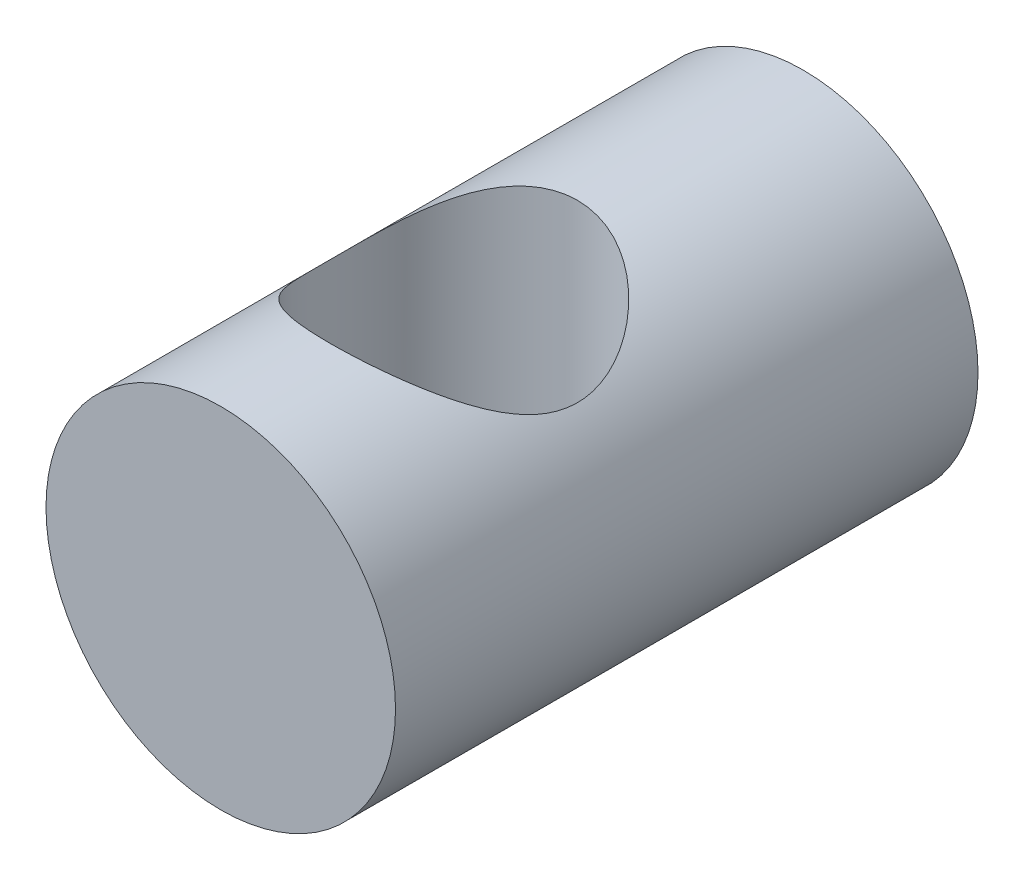
SolidWorks part; units mm, degrees
ref_plane "Front Plane" through (0, 0, 0) normal (0, 0, 1) x (1, 0, 0)
ref_plane "Top Plane" through (0, 0, 0) normal (0, 1, 0) x (1, 0, 0)
ref_plane "Right Plane" through (0, 0, 0) normal (1, 0, 0) x (0, 0, -1)
sketch "Sketch1" plane through (0, 0, 0) normal (0, 0, 1) x (1, 0, 0)
  circle A0 centre (0, 0) radius 6
  dimension "D1" = 12
extrude "Boss-Extrude1" add sketch "Sketch1" along normal blind 20
hole_wizard "M10 Tapped Hole2" positions "Sketch7" profile "Sketch5" tap size "M10" standard "Gb"
sketch "Sketch7" plane through (0, 0, 0) normal (0, 1, 0) x (1, 0, 0)
  line L0 (-6, -20) -> (6, -20) construction
  line L1 (6, -20) -> (6, 0) construction
  point P0 (0, -12)
  dimension "D1" = 8
  dimension "D2" = 6
cosmetic thread "CosmeticThread 2" parameters "D2"=10
sketch "Sketch5" plane through (0, 0, 12) normal (1, 0, 0) x (0, 0, -1)
  line L0 (0, 0) -> (0, 6)
  line L1 (0, 6) -> (4.25, 6)
  line L2 (4.25, 6) -> (4.25, 0)
  line L5 (4.25, 0) -> (0, 0)
  line L11 (0, -6.35) -> (0, 107.95) construction
  dimension "通孔螺纹孔钻头直径" = 8.5
  dimension "通孔螺纹孔钻头深度" = 6
hole_wizard "M10 Tapped Hole1" positions "Sketch9" profile "Sketch8" tap size "M10" standard "Gb"
sketch "Sketch9" plane through (0, 0, 0) normal (0, 1, 0) x (1, 0, 0)
  point P0 (0, -12)
sketch "Sketch8" plane through (0, 0, 12) normal (1, 0, 0) x (0, 0, 1)
  line L0 (0, 0) -> (0, 30.0537)
  line L1 (0, 30.0537) -> (4.25, 27.5)
  line L2 (4.25, 27.5) -> (4.25, 0)
  line L5 (4.25, 0) -> (0, 0)
  line L10 (0, 30.0537) -> (-4.25, 27.5) construction
  line L11 (0, -6.35) -> (0, 107.95) construction
  dimension "螺纹孔钻头直径" = 8.5
  dimension "螺纹孔钻头深度" = 27.5
  dimension "导头角度" = 118
cosmetic thread "CosmeticThread 4"
